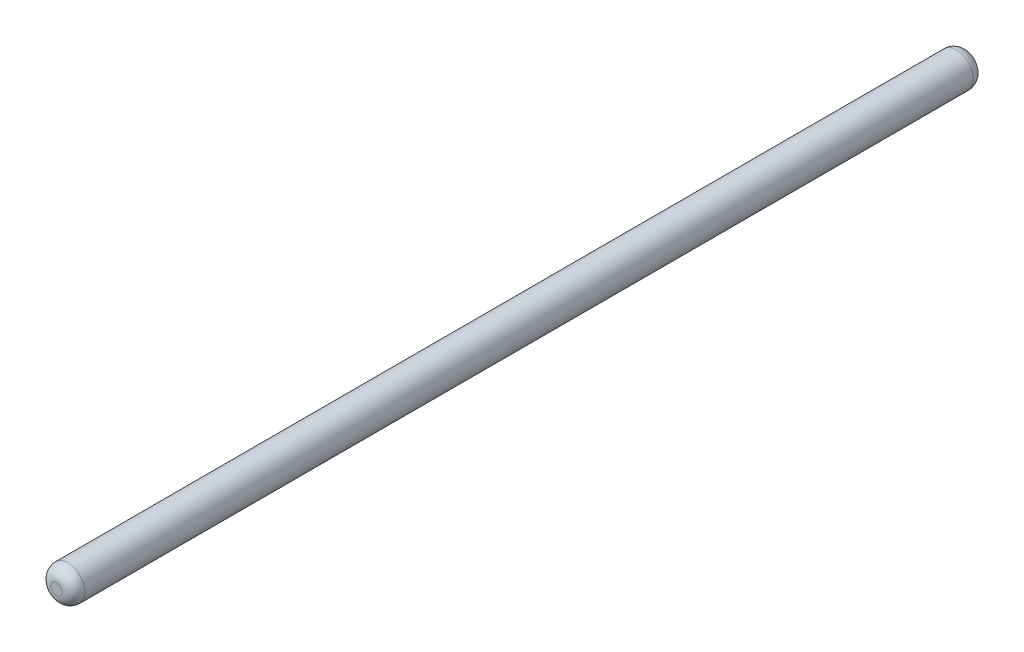
from build123d import *

# Parameters (mm, degrees)
SKETCH1_R           = 0.75
BOSS_EXTRUDE1_DEPTH = 40
FILLET1_R           = 0.5


with BuildPart() as part:
    # Sketch1 → Boss-Extrude1 (new body)
    with BuildSketch(Plane.XY):
        Circle(SKETCH1_R)
    extrude(amount=BOSS_EXTRUDE1_DEPTH)

    # Fillet1
    fillet1_edges = [part.edges().sort_by_distance(p)[0] for p in [
        (-0.75, 0, 0),
        (-0.75, 0, 40),
    ]]
    fillet(fillet1_edges, radius=FILLET1_R)


solid = part.part
